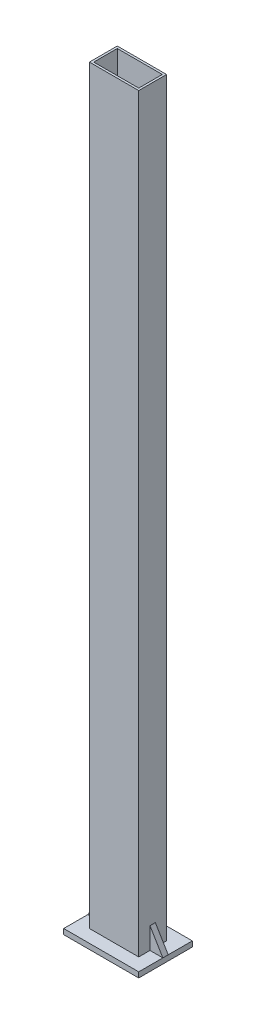
SolidWorks part; units mm, degrees
ref_plane "Front Plane" through (0, 0, 0) normal (0, 0, 1) x (1, 0, 0)
ref_plane "Top Plane" through (0, 0, 0) normal (0, 1, 0) x (1, 0, 0)
ref_plane "Right Plane" through (0, 0, 0) normal (1, 0, 0) x (0, 0, -1)
sketch "Sketch2" plane through (0, 0, 0) normal (0, 1, 0) x (1, 0, 0)
  line L0 (0, 342.2711) -> (0, 0) construction
  line L1 (0, 0) -> (-450, 0) construction
  line L3 (-485, 25) -> (-415, 25)
  line L4 (-485, 25) -> (-485, -25)
  line L5 (-485, -25) -> (-415, -25)
  line L6 (-415, 25) -> (-415, -25)
  line L7 (-485, 25) -> (-415, -25) construction
  line L8 (-485, -25) -> (-415, 25) construction
  dimension "D1" = 450
  dimension "D2" = 70
  dimension "D3" = 50
extrude "Boss-Extrude1" add sketch "Sketch2" along normal blind 5
sketch "Sketch3" plane through (0, 5, 0) normal (0, 1, 0) x (1, 0, 0)
  line L8 (-427, -13) -> (-427, 13)
  line L9 (-427, 13) -> (-473, 13)
  line L10 (-473, 13) -> (-473, -13)
  line L11 (-473, -13) -> (-427, -13)
  line L12 (-427, -13) -> (-427, 13)
  line L13 (-427, 13) -> (-473, 13)
  line L14 (-473, 13) -> (-473, -13)
  line L15 (-473, -13) -> (-427, -13)
  dimension "D1" = 12
extrude "Boss-Extrude2" add sketch "Sketch3" along normal blind 700
sketch "Sketch4" plane through (0, 0, 0) normal (0, 0, 1) x (1, 0, 0)
  line L0 (-473, 5) -> (-485, 5)
  line L1 (-485, 5) -> (-485, 0) construction
  line L2 (-485, 5) -> (-415, 5) construction
  line L3 (-485, 5) -> (-473, 25)
  line L4 (-473, 705) -> (-473, 5) construction
  line L5 (-473, 25) -> (-473, 5)
  line L6 (-450, 0) -> (-450, 13.838) construction
  line L7 (-485, 0) -> (-415, 0) construction
  line L8 (-427, 25) -> (-427, 5)
  line L9 (-415, 5) -> (-427, 25)
  line L10 (-427, 5) -> (-415, 5)
  dimension "D1" = 20
extrude "Boss-Extrude3" add sketch "Sketch4" along normal mid plane 5
sketch "Sketch5" plane through (0, 705, 0) normal (0, 1, 0) x (1, 0, 0)
  line L8 (-471, -11) -> (-429, -11)
  line L9 (-429, -11) -> (-429, 11)
  line L10 (-429, 11) -> (-471, 11)
  line L11 (-471, 11) -> (-471, -11)
  line L12 (-471, -11) -> (-429, -11)
  line L13 (-429, -11) -> (-429, 11)
  line L14 (-429, 11) -> (-471, 11)
  line L15 (-471, 11) -> (-471, -11)
  dimension "D1" = 2
extrude "Cut-Extrude1" cut sketch "Sketch5" against normal blind 691
